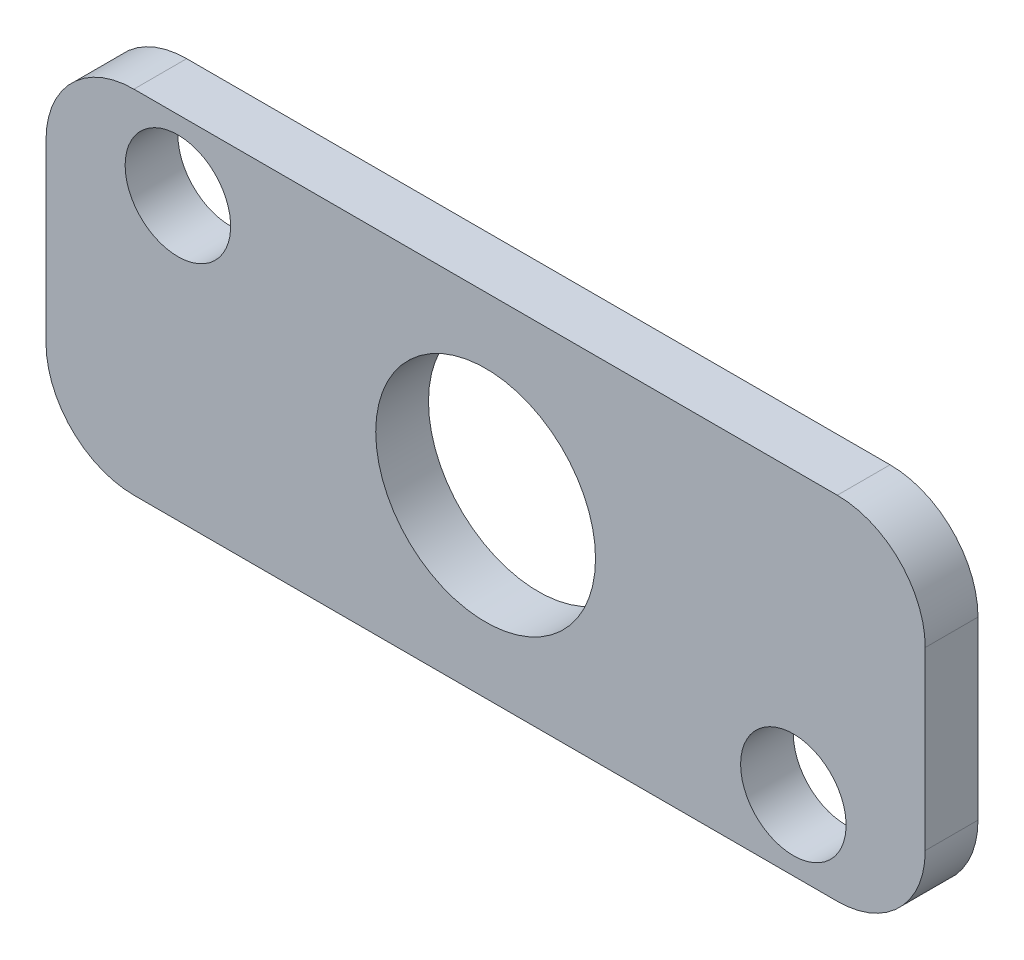
SolidWorks part; units mm, degrees
material "1023 碳钢板 (SS)"
ref_plane "前视基准面" through (0, 0, 0) normal (0, 0, 1) x (1, 0, 0)
ref_plane "上视基准面" through (0, 0, 0) normal (0, 1, 0) x (1, 0, 0)
ref_plane "右视基准面" through (0, 0, 0) normal (1, 0, 0) x (0, 0, -1)
ref_plane "基准面4" through (0, 0, 1.5) normal (0, 0, 1) x (1, 0, 0)
sketch "草图1" plane through (0, 0, 1.5) normal (0, 0, 1) x (1, 0, 0)
  line L0 (-20, -10) -> (20, -10)
  line L1 (25, -5) -> (25, 5)
  line L2 (20, 10) -> (-20, 10)
  line L3 (-25, 5) -> (-25, -5)
  circle A0 centre (-17.5, 6) radius 3
  circle A1 centre (17.5, -6) radius 3
  circle A2 centre (0, 0) radius 6.25
  arc A3 (20, -10) -> (25, -5) centre (20, -5) ccw
  arc A4 (25, 5) -> (20, 10) centre (20, 5) ccw
  arc A5 (-20, 10) -> (-25, 5) centre (-20, 5) ccw
  arc A6 (-25, -5) -> (-20, -10) centre (-20, -5) ccw
extrude "凸台-拉伸1" add sketch "草图1" against normal blind 3
